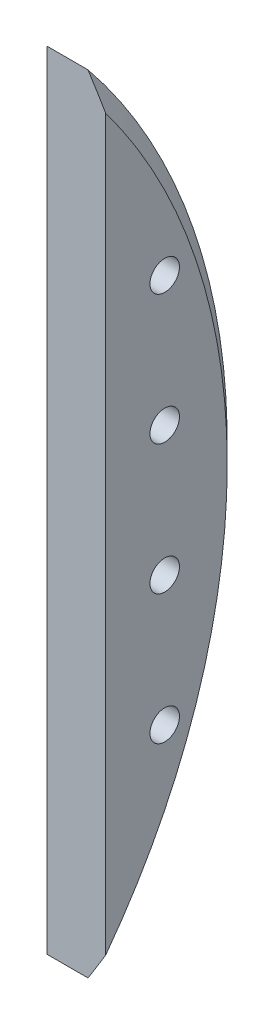
SolidWorks part; units mm, degrees
material "Q235-A"
ref_plane "Front Plane" through (0, 0, 0) normal (0, 0, 1) x (1, 0, 0)
ref_plane "Top Plane" through (0, 0, 0) normal (0, 1, 0) x (1, 0, 0)
ref_plane "Right Plane" through (0, 0, 0) normal (1, 0, 0) x (0, 0, -1)
sketch "Sketch1" plane through (0, 0, 0) normal (1, 0, 0) x (0, 0, -1)
  line L0 (412, 333.4007) -> (412, -333.4007)
  arc A0 (412, -333.4007) -> (412, 333.4007) centre (0, 0) ccw
  dimension "D1" = 1060
  dimension "D2" = 412
extrude "Boss-Extrude1" add sketch "Sketch1" along normal mid plane 50
sketch "Sketch2" plane through (25, 0, 0) normal (1, 0, 0) x (0, 0, -1)
  line L0 (0, 0) -> (462, 0) construction
  line L1 (462, -165) -> (462, 165) construction
  circle A0 centre (462, 55) radius 12.5
  circle A1 centre (462, -55) radius 12.5
  circle A2 centre (462, 165) radius 12.5
  circle A3 centre (462, -165) radius 12.5
  point P6 (462, 0)
  dimension "D1" = 25
  dimension "D2" = 110
  dimension "D3" = 110
  dimension "D4" = 462
extrude "Cut-Extrude1" cut sketch "Sketch2" against normal blind 81
chamfer "Chamfer2" distance 15 angle 45 1 edges at (25, 0, -530)
